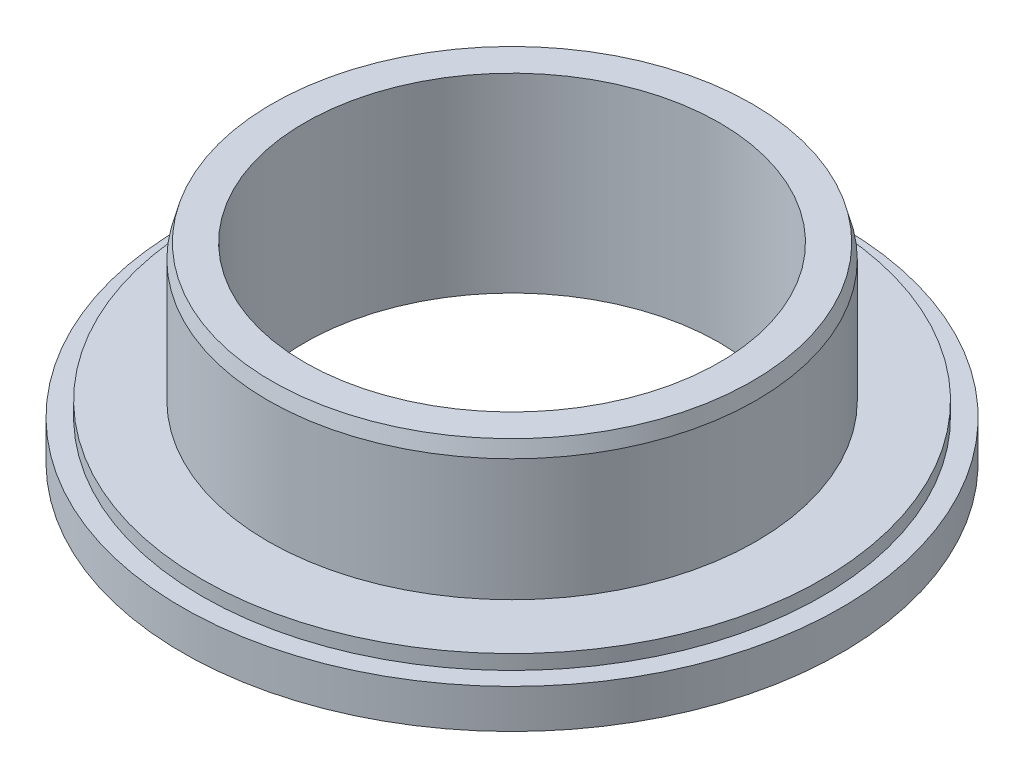
from build123d import *

# Parameters (mm, degrees)
CHAMFER1_SIZE  = 3
CHAMFER1_SIZE2 = 0.803847577


with BuildPart() as part:
    # Sketch1 → Revolve1 (revolve)
    with BuildSketch(Plane.XY, mode=Mode.PRIVATE) as revolve1_sk:
        Polygon((42.5, 31), (50, 31), (50, 3), (63.5, 3), (63.5, 0), (67.5, 0), (67.5, -8), (42.5, -8), align=None)
    revolve(revolve1_sk.sketch.rotate(Axis((0, 0, 0), (0, 1, 0)), 90), axis=Axis((0, 0, 0), (0, 1, 0)))

    # Chamfer1
    chamfer1_edges = [part.edges().sort_by_distance(p)[0] for p in [
        (0, 31, 50),
    ]]
    chamfer1_side = [part.faces().sort_by_distance(p)[0] for p in [
        (0, 17, 50),
    ]]
    chamfer(chamfer1_edges, length=CHAMFER1_SIZE, length2=CHAMFER1_SIZE2, reference=chamfer1_side[0])


solid = part.part
